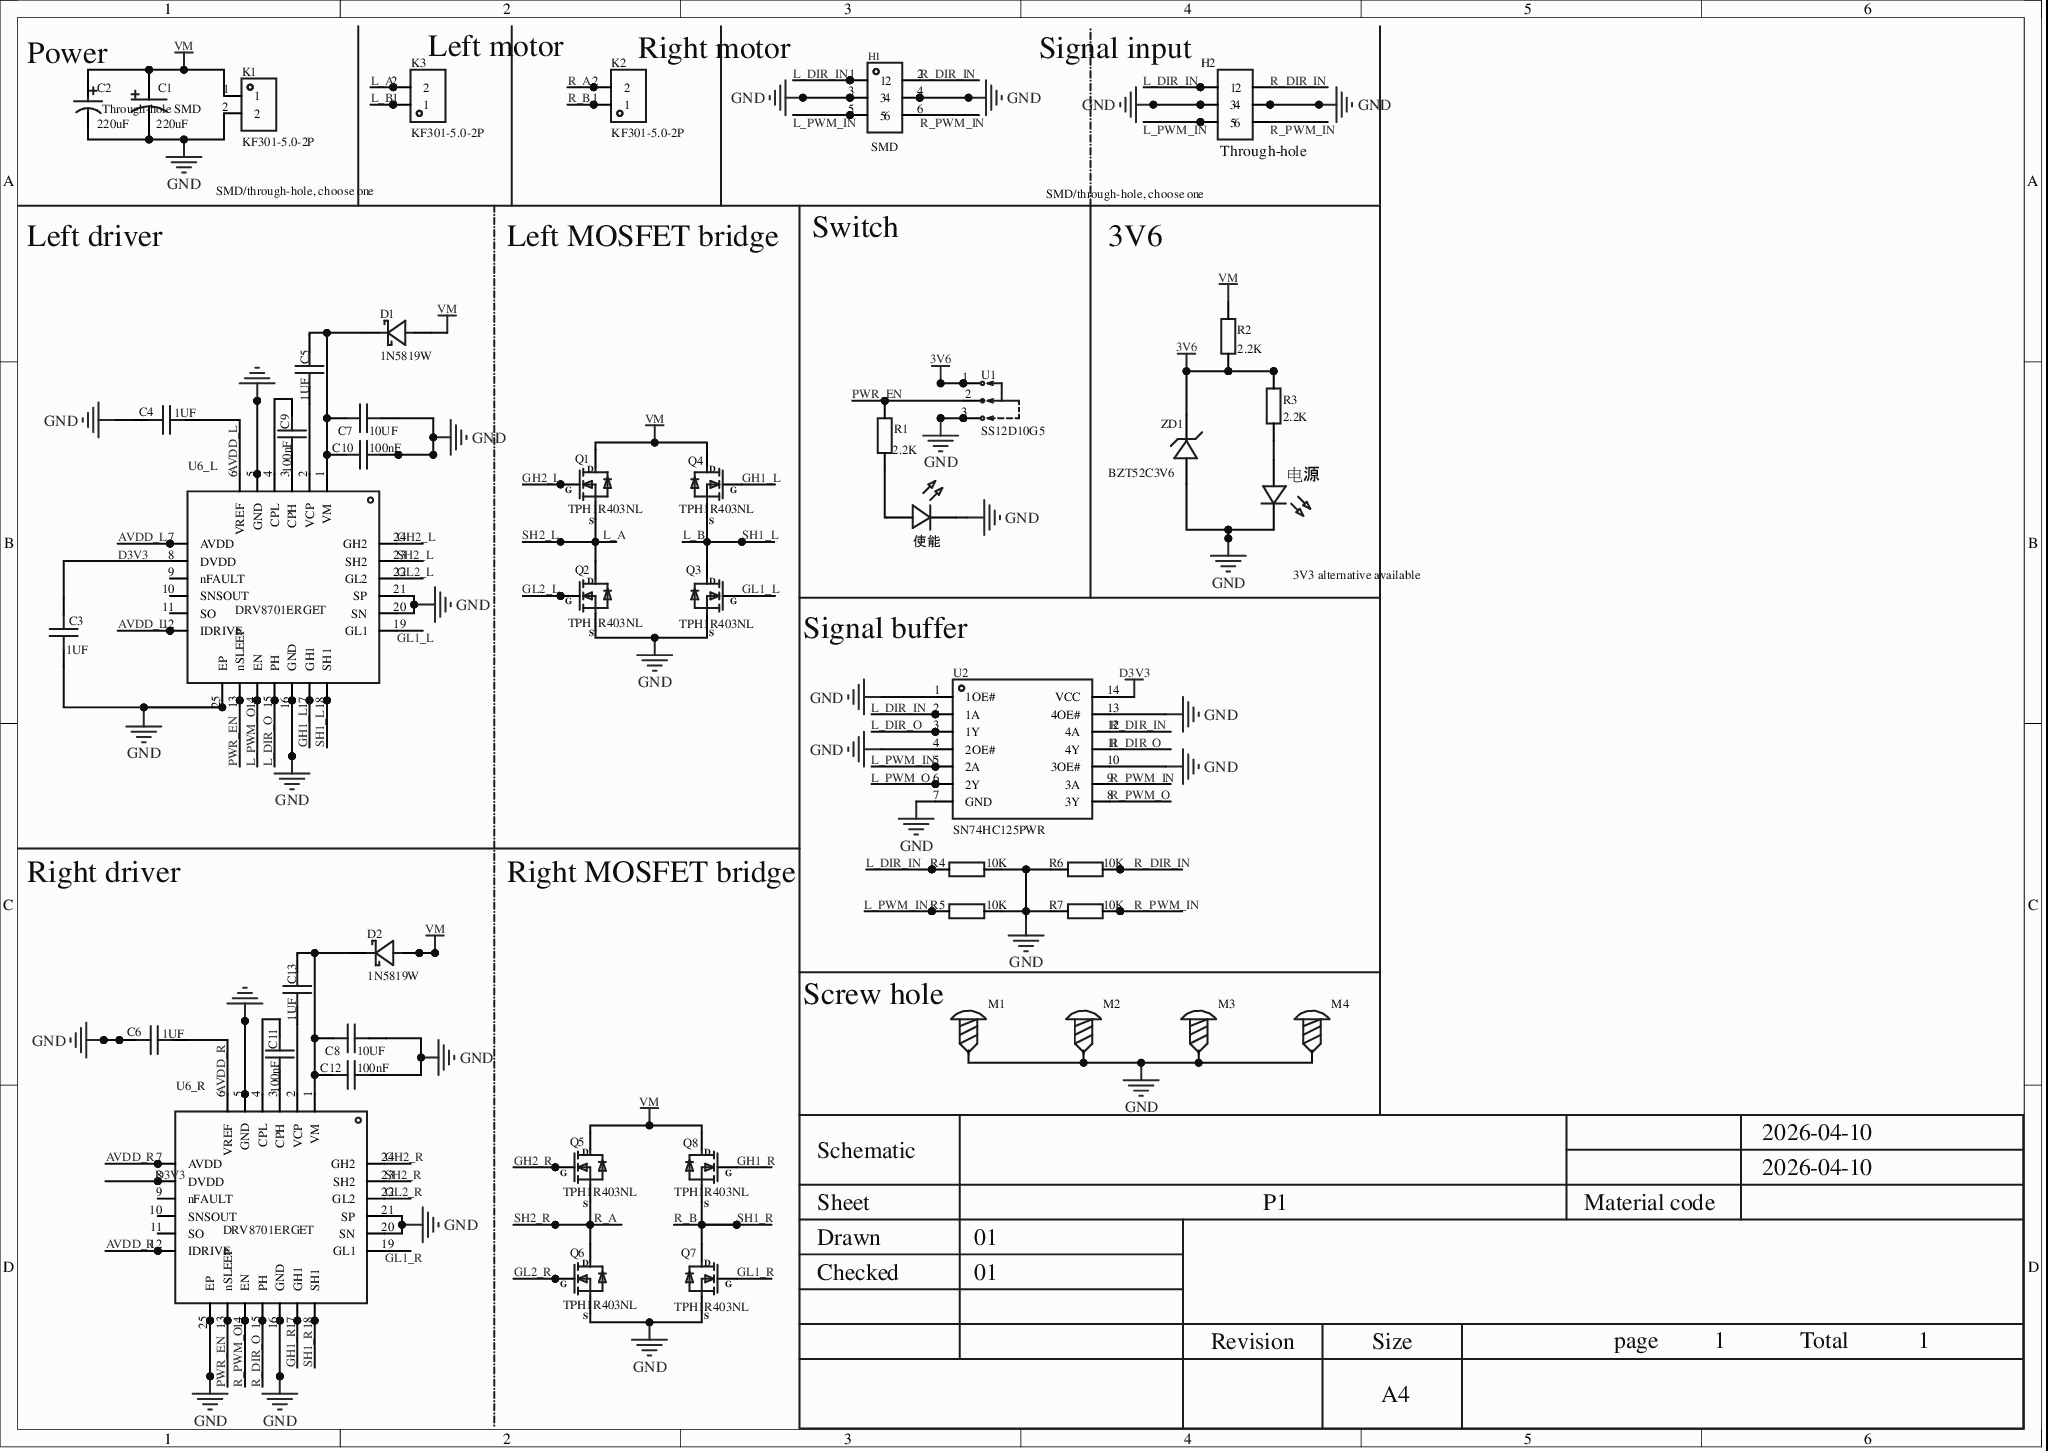
[diagram p0: MISC62357-3.schdoc]
# Altium project MISC62357-2.PrjPcb
1 sheet, 46 parts. Net scope: global (net labels, ports and power ports of the same name join across sheets).
Board file: MISC62357.pcbdoc

## Sheet MISC62357-3.schdoc
size 297 x 210 mm; Version: V1.0; @Project Name: MISC62357; @Page Count: 1; @Update Date: 2026-04-10; @Create Date: 2026-04-10; @Schematic Name: MISC62357; @Page No: 1; @Board Name: MISC62357; @Create Time: 08:46:51; @Update Time: 16:46:51

### Parts
C1  220uF  [CAP-SMD_BD8.0-L8.3-W8.3-FD]
C2  220uF  [CAP-TH_BD8.0-P3.50-D0.6-FD]
C3  1UF  [C0603]
C4  1UF  [C0603]
C5  1UF  [C0603]
C6  1UF  [C0603]
C7  10UF  [C0603]
C8  10UF  [C0603]
C9  100nF  [C0603]
C10  100nF  [C0603]
C11  100nF  [C0603]
C12  100nF  [C0603]
C13  1UF  [C0603]
D1  1N5819W  [SOD-123_L2.7-W1.6-LS3.7-RD-1]
D2  1N5819W  [SOD-123_L2.7-W1.6-LS3.7-RD-1]
H1  SMD  [HDR-SMD_6P-P2.54-V-M-R2-C5-S7.4]
H2  (no value)  [HDR-TH_6P-P2.54-V-R2-C3-S2.54_A2541WV-2X3P]
K1  KF301-5.0-2P  [CONN-TH_P5.00_KF301-5.0-2P]
K2  KF301-5.0-2P  [CONN-TH_P5.00_KF301-5.0-2P]
K3  KF301-5.0-2P  [CONN-TH_P5.00_KF301-5.0-2P]
M1  (no value)  [M4螺丝]
M2  (no value)  [M4螺丝]
M3  (no value)  [M4螺丝]
M4  (no value)  [M4螺丝]
Q1  TPH1R403NL  [DFN5x6]
Q2  TPH1R403NL  [DFN5x6]
Q3  TPH1R403NL  [DFN5x6]
Q4  TPH1R403NL  [DFN5x6]
Q5  TPH1R403NL  [DFN5x6]
Q6  TPH1R403NL  [DFN5x6]
Q7  TPH1R403NL  [DFN5x6]
Q8  TPH1R403NL  [DFN5x6]
R1  2.2K  [R0603]
R2  2.2K  [R0603]
R3  2.2K  [R0603]
R4  10K  [R0603]
R5  10K  [R0603]
R6  10K  [R0603]
R7  10K  [R0603]
U1  SS12D10G5  [SW-TH_SHOU-HAN_SS12D10G4]
U2  SN74HC125PWR  [TSSOP-14_L5.0-W4.4-P0.65-LS6.5-BL]
U6_L  DRV8701ERGET  [VQFN-24_L4.0-W4.0-P0.50-BL-EP2.5]
U6_R  DRV8701ERGET  [VQFN-24_L4.0-W4.0-P0.50-BL-EP2.5]
ZD1  BZT52C3V6  [SOD-123_L2.8-W1.8-LS3.7-RD]
使能  (no value)  [LED_0603]
电源  (no value)  [LED_0603]

### Nets
3V6: R2.1 R3.2 U1.1 ZD1.1(K)
D3V3: C3.2 U2.14(VCC) U6_L.8(DVDD) U6_R.8(DVDD)
GND: C1.2 C2.2 C3.1 C4.2 C6.2 C7.2 C8.2 C10.2 C12.2 H1.3 H1.4 H2.3 H2.4 K1.2 M1.1 M2.1 M3.1 M4.1 Q2.3(S) Q3.3(S) Q6.3(S) Q7.3(S) R4.2 R5.2 R6.1 R7.1 U1.3 U2.1(1OE#) U2.4(2OE#) U2.7(GND) U2.10(3OE#) U2.13(4OE#) U6_L.5(GND) U6_L.16(GND) U6_L.20(SN) U6_L.21(SP) U6_L.25(EP) U6_R.5(GND) U6_R.16(GND) U6_R.20(SN) U6_R.21(SP) U6_R.25(EP) ZD1.2(A) 使能.1(C) 电源.1(C)
VM: C1.1 C2.1 D1.2(A) D2.2(A) K1.1 Q1.1(D) Q4.1(D) Q5.1(D) Q8.1(D) R2.2
AVDD_L: C4.1 U6_L.6(VREF) U6_L.7(AVDD) U6_L.12(IDRIVE)
AVDD_R: C6.1 U6_R.6(VREF) U6_R.7(AVDD) U6_R.12(IDRIVE)
GH1_L: Q4.2(G) U6_L.17(GH1)
GH1_R: Q8.2(G) U6_R.17(GH1)
GH2_L: Q1.2(G) U6_L.24(GH2)
GH2_R: Q5.2(G) U6_R.24(GH2)
GL1_L: Q3.2(G) U6_L.19(GL1)
GL1_R: Q7.2(G) U6_R.19(GL1)
GL2_L: Q2.2(G) U6_L.22(GL2)
GL2_R: Q6.2(G) U6_R.22(GL2)
L_A: K3.2 Q1.3(S) Q2.1(D) U6_L.23(SH2)  [also labelled SH2_L]
L_B: K3.1 Q3.1(D) Q4.3(S) U6_L.18(SH1)  [also labelled SH1_L]
L_DIR_IN: H1.1 H2.1 R4.1 U2.2(1A)
L_DIR_O: U2.3(1Y) U6_L.15(PH)
L_PWM_IN: H1.5 H2.5 R5.1 U2.5(2A)
L_PWM_O: U2.6(2Y) U6_L.14(EN)
PWR_EN: R1.2 U1.2 U6_L.13(nSLEEP) U6_R.13(nSLEEP)
R_A: K2.2 Q5.3(S) Q6.1(D) U6_R.23(SH2)  [also labelled SH2_R]
R_B: K2.1 Q7.1(D) Q8.3(S) U6_R.18(SH1)  [also labelled SH1_R]
R_DIR_IN: H1.2 H2.2 R6.2 U2.12(4A)
R_DIR_O: U2.11(4Y) U6_R.15(PH)
R_PWM_IN: H1.6 H2.6 R7.2 U2.9(3A)
R_PWM_O: U2.8(3Y) U6_R.14(EN)
NetC5_1: C5.1 C7.1 C10.1 D1.1(K) U6_L.1(VM)
NetC5_2: C5.2 U6_L.2(VCP)
NetC8_1: C8.1 C12.1 C13.1 D2.1(K) U6_R.1(VM)
NetC9_1: C9.1 U6_L.3(CPH)
NetC9_2: C9.2 U6_L.4(CPL)
NetC11_1: C11.1 U6_R.3(CPH)
NetC11_2: C11.2 U6_R.4(CPL)
NetC13_2: C13.2 U6_R.2(VCP)
NetR1_1: R1.1 使能.2(A)
NetR3_1: R3.1 电源.2(A)

Not connected (* = marked no-connect by the designer): U6_L 9(nFAULT)* 10(SNSOUT)* 11(SO)*; U6_R 9(nFAULT)* 10(SNSOUT)* 11(SO)*

### Notes on the sheet
- (near C2) Power
- Left motor
- (near K2) Right motor
- (near H2) Signal input
- (near C1) Through-hole
- (near C1) SMD
- (near H2) Through-hole
- Left driver
- SMD/through-hole, choose one
- Left MOSFET bridge
- Switch
- (near H2) SMD/through-hole, choose one
- 3V6
- (near 电源) 3V3 alternative available
- Signal buffer
- Right driver
- Right MOSFET bridge
- Screw hole
- 2026-04-10
- Schematic
- Sheet
- P1
- Material code
- Checked
- Drawn
- 01
- Revision
- Size
- A4
- page
- 1
- Total

### Library data of the parts
C1 = EEEFT1H221GP: Capacitance:220uF;Tolerance:±20%;Rated voltage:50V;Ripple current:670mA@100kHz;ESR:180mΩ@100kHz;; Manufacturer: PANASONIC(松下); AddInBom: yes; Tolerance: ±20%; Rated Voltage: 50V; φD: 8mm; L: 10.5mm; Lifetime @ Temp: 5000hrs@105℃; ModelId: 5c9301d64f8b45ea89e061ac72e6cbf7; ModelTransform: 393.7,326.771,0,180,0,0,0,0,0; Device: EEEFT1H221GP; Symbol: EEEFT1H221GP; Supplier: LCSC; Supplier Part: C178595; Manufacturer Part: EEEFT1H221GP; Value: 220uF; JLCPCB Part Class: Extended library; FootprintName: CAP-SMD_BD8.0-L8.3-W8.3-FD; LCSC Part Name: 220uF ±20% 50V; Supplier Footprint: SMD,D8xL10.2mm; Datasheet: example.com/20180420/C190724_5C30A39F6DC8D73DF4133310F276C40B.pdf; ConvertToPcb: yes; Ripple Current: 670mA@100kHz; Equivalent Series Resistance(ESR): 180mΩ@100kHz; Operating Temperature: -55℃~+105℃; ModelName: CAP-SMD_BD8.0-L8.3-W8.3-FD
C2 = ERS1VM221F12OT: Capacitance:220uF;Tolerance:±20%;Rated voltage:35V;; Manufacturer: AISHI(艾华集团); AddInBom: yes; Tolerance: ±20%; Rated Voltage: 35V; φD: 8mm; L: 12mm; Lifetime @ Temp: 7000hrs@105℃; ModelId: a2c936ec27754f809f3966430e36f767; ModelName: CAP-TH_D8.0-H8.0-P3.50; ModelTransform: 314.96,314.862,0,180,0,0,0,0,-137.795; Device: ERS1VM221F12OT; Symbol: ERS1VM221F12OT; FootprintName: CAP-TH_BD8.0-P3.50-D0.6-FD; LCSC Part Name: 220uF ±20% 35V; SupplierPart: C106697; ManufacturerPart: ERS1VM221F12OT; Supplier Footprint: 插件,D8xL12mm; JLCPCB Part Class: Extended library; Datasheet: example.com/20191015/C438940_4B8E60A742BB0AE40DDEF87A5C89089D.pdf; Supplier: LCSC; ConvertToPcb: yes; Value: 220uF; Lead Spacing: 3.5mm
C3-C13 = CAP_0603: SymbolName: CapAcitance; ConvertToPcb: yes; ModelId: ac125912035d415993ca9572d50418b1; ModelName: C0603_L1.6-W0.8-H0.8; ModelTransform: 62.992,31.496,0,0,0,0,0,0,0; Device: CAP_0603; FootprintName: C0603; AddInBom: yes; Supplier Footprint: 0603
  C3-C6 C13: Value: 1UF
  C7 C8: Value: 10UF
  C9-C12: Value: 100nF
D1 D2 = 1N5819W: Diode configuration:-;Forward voltage (Vf):900mV@3A;DC reverse voltage (Vr):40V;Average rectified current (Io):1A;; Manufacturer: TECH PUBLIC(台舟); Symbol: 1N5819W_C2905650; AddInBom: yes; Reverse Voltage (Vr): 40V; Average Rectified Current (Io): 1A; Reverse Leakage Current (Ir): 1mA@40V; ModelId: 528459655f7d4601a76356f3191c812b; ModelTransform: 151.575,66.929,0,0,0,0,0,0,0; Device: 1N5819W; FootprintName: SOD-123_L2.7-W1.6-LS3.7-RD-1; LCSC Part Name: 电压:40V 电流:1A; SupplierPart: C2905650; ManufacturerPart: 1N5819W; Supplier Footprint: SOD-123; JLCPCB Part Class: Extended library; Datasheet: example.com/20211020/7FEA34DA99E5285CBA3CC87767B82BE7.pdf; Supplier: LCSC; ConvertToPcb: yes; Diode Configuration: -; Forward Voltage (Vf@If): 900mV@3A; ModelName: SOD-123_L2.7-W1.6-LS3.7-RD-1
H1 = 2.54-2*3P立贴针: Pin structure:-;Pitch:2.54mm;Row spacing:-;Round/square pin:-;Mounting type:-;Rows:double row;Total pins:6P;Rated current:-;Rated voltage:-;Mating pin length:-;Plastic height:-;Contact material:-;Contact plating:-;Color:black;; Manufacturer Part: 贴片; Manufacturer: BOOMELE(博穆精密); Device: 2.54-2*3P vertical SMD header; AddInBom: yes; Pitch: 2.54mm; ModelId: 04f7a77b3a774fdf8b1caeaa3d5fc986; ModelName: HDR-SMD_6P-P2.54-M-LS-2X3P; ModelTransform: 299.9994,275.59,0,0,0,0,0,0.001,0; Symbol: 2.54-2*3P vertical SMD header; Supplier: LCSC; Supplier Part: C192301; JLCPCB Part Class: Extended library; FootprintName: HDR-SMD_6P-P2.54-V-M-R2-C5-S7.4; LCSC Part Name: 间距:2.54mm; Supplier Footprint: SMD,P=2.54mm,卧贴; ConvertToPcb: yes; Pin Structure: -; Row Spacing: -; Circluar Pins/Square Pins: -; Mounting Type: -; Number of Rows: Double row; Number of Pins: 6P; Current Rating (Max): -; Voltage Rating (Max): -; Length of Mating Pin: -; Insulation Height: -; Contact Material: -; Contact Plating: -; Color: Black
H2 = HDR-M_2.54_2x3: Symbol: HDR-M-2.54_2x3; ConvertToPcb: yes; ModelId: fd1b55b786fb415ca65c4187088147b7; ModelName: HDR2.54-M-LI-2x3P; ModelTransform: 299.9994,200,0,0,0,0,0,0,-118.11; Device: HDR-M_2.54_2x3; FootprintName: HDR-TH_6P-P2.54-V-R2-C3-S2.54_A2541WV-2X3P; AddInBom: yes; SupplierPart: C402781; Supplier Footprint: 插件,P=2.54mm
K1 = KF301-5.0-2P: Structure:1x2P;Pitch:5mm;Color:blue;Mounting:through-hole;Rated current:17A;Rated voltage:250V;Rows:1;Wire gauge - AWG:14~22;Wire gauge - mm2:1.5;Pins per row:2;Operating temperature:-30℃~+120℃;; Manufacturer: KEFA(科发); AddInBom: yes; Structure: 1x2P; Pitch: 5mm; Current Rating (Max): 17A; Voltage Rating (Max): 250V; Wire Gauge - AWG: 14~22; Wire Gauge - mm2: 1.5; Number of PINs Per Row: 2; ModelId: 442de893d0fc4728b9e5c7abc29ccda5; ModelTransform: 409.448,303.149,0,0,0,0,7.874,5.906,-169.291; Device: KF301-5.0-2P; Symbol: KF301-5.0-2P; Supplier: LCSC; Supplier Part: C474881; Manufacturer Part: KF301-5.0-2P; JLCPCB Part Class: Extended library; FootprintName: CONN-TH_P5.00_KF301-5.0-2P; LCSC Part Name: 5mm 1x2P 排数:1 每排P数:2 直插; Supplier Footprint: 插件,P=5mm; Datasheet: example.com/20230317/03A5B5FC229D6F9225E8F51DA1A4E80A.pdf; ConvertToPcb: yes; Color: Blue; Mounting Style: Through-hole; Number of Pins: 2P; Number of Rows: 1; Operating Temperature Range: -30℃~+120℃; ModelName: CONN-TH_P5.00_KF301-5.0-2P
K2 K3 = KF301-5.0-2P: Structure:1x2P;Pitch:5mm;Color:blue;Mounting:through-hole;Rated current:17A;Rated voltage:250V;Rows:1;Wire gauge - AWG:14~22;Wire gauge - mm2:1.5;Pins per row:2;Operating temperature:-30℃~+120℃;; Manufacturer: KEFA(科发); 3D Model: 442de893d0fc4728b9e5c7abc29ccda5; 3D Model Transform: 409.448,303.149,0,0,0,0,7.874,5.906,-169.291; Structure: 1x2P; Pitch: 5mm; Current Rating (Max): 17A; Voltage Rating (Max): 250V; Wire Gauge - AWG: 14~22; Wire Gauge - mm2: 1.5; Number of PINs Per Row: 2; AddInBom: yes; Device: KF301-5.0-2P; Symbol: KF301-5.0-2P; LCSC Part Name: 5mm 1x2P 排数:1 每排P数:2 直插; Supplier Footprint: 插件,P=5mm; Datasheet: example.com/20230317/03A5B5FC229D6F9225E8F51DA1A4E80A.pdf; Color: Blue; Mounting Style: Through-hole; Number of Pins: 2P; Number of Rows: 1; Operating Temperature Range: -30℃~+120℃; Supplier: LCSC; Supplier Part: C474881; Manufacturer Part: KF301-5.0-2P; JLCPCB Part Class: Extended library; FootprintName: CONN-TH_P5.00_KF301-5.0-2P; ConvertToPcb: yes; ModelName: CONN-TH_P5.00_KF301-5.0-2P
M1-M4 = M4螺丝: Device: M4 screw; Symbol: Screw hole; ConvertToPcb: yes; FootprintName: M4 screw; AddInBom: yes; Supplier Footprint: 插件
Q1-Q8 = TPH1R403NL: AddInBom: yes; ModelId: 2220501111284f4fa264999823e2c1e0; ModelName: PDFN5x6; ModelTransform: 196.85,238.1885,38.9763,0,0,0,0,0,0; Device: TPH1R403NL; SymbolName: TPH1R403NL; ConvertToPcb: yes
R1-R7 = Res_0603: Symbol: Resistor; ConvertToPcb: yes; ModelId: fc143cca1e79419f9cd78b61e9279f08; ModelTransform: 31.8897,63.7794,0,90,0,0,0,0,0; Device: Res_0603; FootprintName: R0603; AddInBom: yes; Supplier Footprint: 0603; ModelName: R0603
  R1-R3: Value: 2.2K
  R4-R7: Value: 10K
U1 = SS12D10G5: 电路结构:单刀双掷;安装方式:直插;额定电流(DC):2A;额定电压(DC):125V;机械寿命:3千次;; Manufacturer: SHOU HAN(首韩); AddInBom: yes; Circuit: SPDT; Switch Length: 12.7mm; Switch Width: 6.7mm; Current Rating (DC): 2A; Voltage Rating (DC): 125V; Mechanical Life: 3千次; ModelId: cfce8581009a45839cc96a3fa85751f8; ModelTransform: 499.999,263.779,0,0,0,0,-0.589,-0.591,-196.85; Device: SS12D10G5; Symbol: SS12D10G5; FootprintName: SW-TH_SHOU-HAN_SS12D10G4; LCSC Part Name: 两档立式插件 3脚拨动开关 柄长5.0mm; SupplierPart: C7431054; ManufacturerPart: SS12D10G5; Supplier Footprint: 插件; JLCPCB Part Class: Extended library; Datasheet: example.com/20231130/7A3DB6A149BF0A1DCFFE64FFC07FE434.pdf; Supplier: LCSC; ConvertToPcb: yes; Mounting Style: Through-hole; Operating Temperature: -25℃~+70℃; ModelName: SW-TH_SHOU-HAN_SS12D10G4
U2 = SN74HC125PWR: Input type:-;Supply voltage:2V~6V;Number of elements:4;Bits per element:1;Sink current (IOL):7.8mA;Source current (IOH):7.8mA;; Manufacturer: TI(德州仪器); AddInBom: yes; output type: Tri-state; Supply Voltage: 2V~6V; Number of Elements: 4; Number of Bits per Element: 1; Sink Current: 7.8mA; Logic Family: 74HC; ModelId: 02f1f60386074b2ca8e111040ac061f2; ModelName: TSSOP-14_L5.0-W4.4-H1.0-LS6.4-P0.65; ModelTransform: 236.714,196.85,0,90,0,0,0,0,0; Device: SN74HC125PWR; Symbol: SN74HC125PWR; FootprintName: TSSOP-14_L5.0-W4.4-P0.65-LS6.5-BL; LCSC Part Name: SN74HC125PWR; SupplierPart: C132994; ManufacturerPart: SN74HC125PWR; Supplier Footprint: TSSOP-14; JLCPCB Part Class: Extended library; Supplier: LCSC; ConvertToPcb: yes; Input type: -; Source Current: 7.8mA; Operating Temperature: -40℃~+85℃
U6_L U6_R = DRV8701ERGET: DRV8701 47V H-bridge smart gate driver; Manufacturer: TI(德州仪器); AddInBom: yes; ModelId: 12827167658848359cc215f26847ede4; ModelName: VQFN-24_L4.0-W4.0-H1.0-P0.50-BL-EP2.5; ModelTransform: 157.48,157.48,0,90,0,0,-0.001,0.001,0; Device: DRV8701ERGET; Symbol: DRV8701ERGET; FootprintName: VQFN-24_L4.0-W4.0-P0.50-BL-EP2.5; LCSC Part Name: 有刷直流电机驱动芯片 5.5V; SupplierPart: C132049; ManufacturerPart: DRV8701ERGET; Supplier Footprint: VQFN-24(4x4); JLCPCB Part Class: Extended library; Supplier: LCSC; ConvertToPcb: yes
ZD1 = BZT52C3V6_C2113: Diode configuration:single;Zener voltage (nominal):3.6V;Zener voltage (range):3.4V~3.8V;Power:350mW;Tolerance:-;; Manufacturer: CJ(江苏长电/长晶); AddInBom: yes; Diode Configuration: Single; Zener Voltage (Nom): 3.6V; Reverse Leakage Current (Ir): 5uA@1V; Power Dissipation: 350mW; Zener Impedance (Zzt): 90Ω; ModelId: 7884390a25fb4c08947731ebfba7e3f8; ModelTransform: 144.8816,62.992,0,0,0,0,0,0,0; Device: BZT52C3V6_C2113; Symbol: BZT52C3V6_C2113; FootprintName: SOD-123_L2.8-W1.8-LS3.7-RD; LCSC Part Name: BZT52C3V6; SupplierPart: C2113; ManufacturerPart: BZT52C3V6; Supplier Footprint: SOD-123; JLCPCB Part Class: Extended library; Datasheet: example.com/20140508/1457707057629.pdf; Supplier: LCSC; ConvertToPcb: yes; Zener Voltage (Range): 3.4V~3.8V; Tolerance: -; ModelName: SOD-123_L2.8-W1.8-LS3.7-RD
使能 = LED_0603-G: Symbol: LED_G; Convert to PCB: yes; 3D Model: 8b5fcaf0229049f8a37a9c352bb0ca0a; 3D Model Transform: 63.1,31.6,23.7,0,0,0,0,0,0; ModelName: LED-0603_G; Device: LED_0603-G; Add into BOM: yes; Supplier Footprint: 0603; FootprintName: LED_0603
电源 = LED_0603-R: Symbol: LED_R; Convert to PCB: yes; 3D Model: dd8257b0d61a4cd7b68939a056e08095; 3D Model Transform: 58.72,29.4,22.03,0,0,0,0,0,0; ModelName: LED-0603_R; Device: LED_0603-R; Add into BOM: yes; Supplier Footprint: 0603; FootprintName: LED_0603